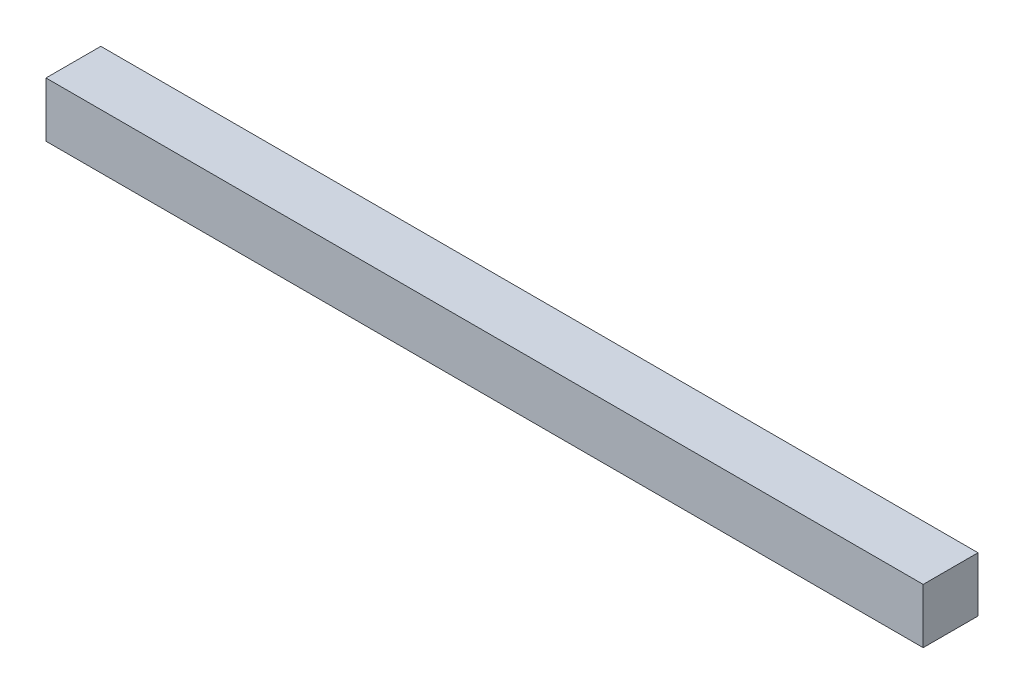
SolidWorks part; units mm, degrees
ref_plane "前视基准面" through (0, 0, 0) normal (0, 0, 1) x (1, 0, 0)
ref_plane "上视基准面" through (0, 0, 0) normal (0, 1, 0) x (1, 0, 0)
ref_plane "右视基准面" through (0, 0, 0) normal (1, 0, 0) x (0, 0, -1)
sketch "草图1" plane through (0, 0, 0) normal (0, 0, 1) x (1, 0, 0)
  line L1 (0, 0) -> (80, 0)
  line L2 (0, 0) -> (0, 5)
  line L3 (0, 5) -> (80, 5)
  line L4 (80, 0) -> (80, 5)
extrude "凸台-拉伸1" add sketch "草图1" along normal blind 5
